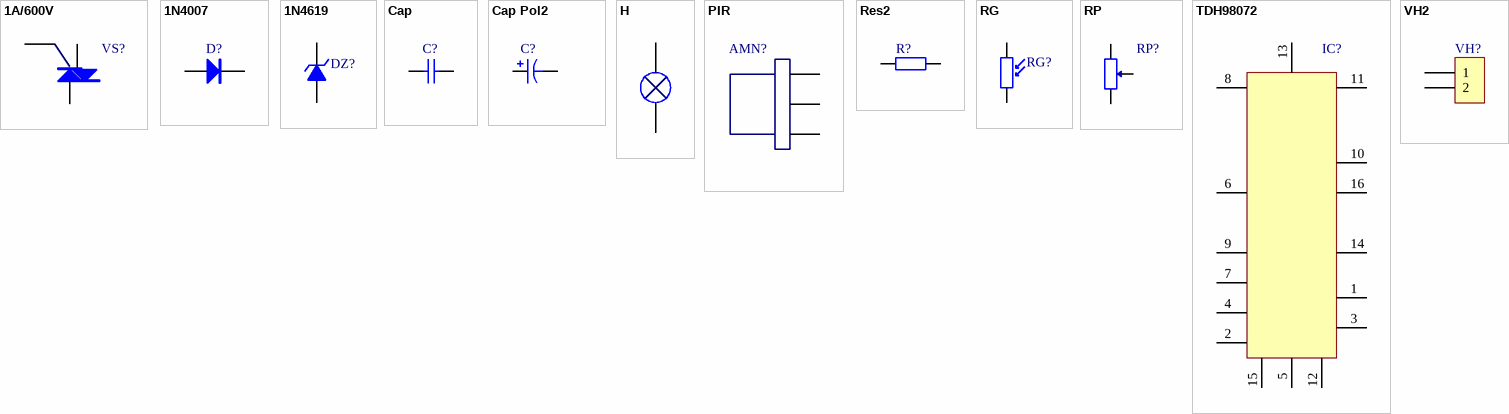
[diagram p0: symbols 1A/600V to VH2]
# Altium schematic symbol library MISC82068-5.SCHLIB: 12 symbols
Pins are listed as number, name and electrical type; pins without a type are passive.


## 1A/600V
designator VS?
footprint DO-41 (2.6*9.1mm (diameter, lead spacing))
footprint SOD-123 (2.7x1.6X1.1mm (L x W x H, excluding leads))
footprint SMA (4.5x2.6*2.2mm (L x W x H, excluding leads))
footprint DO-41V (2.6*3.5mm (diameter, lead spacing))
footprint LED 3mm-2P (3mm bicolour LED)
pins: 1, 2, 3

## 1N4007
designator D?
Rectifier diode
footprint DO-41 (2.6*9.1mm (diameter, lead spacing))
footprint SOD-123 (2.7x1.6X1.1mm (L x W x H, excluding leads))
footprint SMA (4.5x2.6*2.2mm (L x W x H, excluding leads))
footprint DO-41V (2.6*3.5mm (diameter, lead spacing))
pins: 1 A, 2 K

## 1N4619
designator DZ?
3V/0.5W Zener diode
footprint DO-35 (1.8*6.8mm (diameter, lead spacing))
footprint MINI_MELF (LL34) (1.5*3.4mm (diameter, lead spacing))
footprint DO-35V (1.8*2.5mm (diameter, lead spacing))
pins: 1 A, 2 K

## Cap
designator C?
Capacitor
footprint RAD-0.3 (Radial Cap, Thru-Hole; 2 Leads; 0.3 in Pin Spacing)
simulation model CAP (Capacitor)
signal-integrity model Cap
pins: 1, 2

## Cap Pol2
designator C?
Polarized Capacitor (Axial)
footprint POLAR0.8 (Polarized Capacitor; 2 Leads)
simulation model CAP (Capacitor)
signal-integrity model Cap Pol
pins: 1, 2
1 alternate drawing of the same symbol

## H
designator *?
footprint HDR1X2 (Connector; Header; 2 Position)
pins: 1, 2

## PIR
designator AMN?
footprint HDR1X3 (Connector; Header; 3 Position)
pins: 1, 2, 3

## Res2
designator R?
Resistor
footprint AXIAL-0.4 (Axial Device, Thru-Hole; 2 Leads; 0.4 in Pin Spacing)
simulation model RESISTOR (Resistor)
signal-integrity model Res
pins: 1, 2

## RG
designator RG?
Photoresistor
footprint RG5528 (Photoresistor, pin pitch: 3mm)
footprint AXIAL-0.4 (Axial Device, Thru-Hole; 2 Leads; 0.4 in Pin Spacing)
pins: 1, 2

## RP
designator RP?
Single potentiometer
footprint 3296W (Precise Multi-Winding Adjustable Resistor)
footprint 3306W
footprint 3319P
footprint 3362P
footprint 3386W
footprint RM065 (Blue-white adjustable potentiometer)
footprint WH148-1-G15 (Single potentiometer, pin pitch: 5mm, shaft length: 15mm)
footprint WH148-1-G18 (Single potentiometer, pin pitch: 5mm, shaft length: 18mm)
footprint WH148-1-G20 (Single potentiometer, pin pitch: 5mm, shaft length: 20mm)
footprint WH148-1-G25 (Single potentiometer, pin pitch: 5mm, shaft length: 25mm)
footprint 3266W (L: 7mm, W: 4.8mm, H: 7.5mm)
footprint 3266X (L: 7mm, W: 4.8mm, H: 7.5mm)
footprint 3266Y (L: 7mm, W: 4.8mm, H: 7.5mm)
footprint 3266Z (L: 7mm, W: 4.8mm, H: 7.5mm)
footprint XV09223NPV-20F (L 9.85mm, W 11.55mm, H 20mm)
footprint XV09223NPV-25F (L 9.85mm, W 11.55mm, H 25mm)
footprint XV09223NPV-30F (L 9.85mm, W 11.55mm, H 30mm)
footprint 3006P (19.05mm*4.83mm*6.35mm (L*W*H))
pins: 1, 2, 3

## TDH98072
designator IC?
footprint DIP16
pins: 1 VSS, 2 VSS, 3 VSS, 4 VSS, 5 VSS, 6 VSS, 7 VSS, 8 VSS, 9 VSS, 10 VSS, 11 VSS, 12 VSS, 13 VSS, 14 VSS, 15 VSS, 16 VSS

## VH2
designator VH?
footprint VH3.96-2A
footprint VH3.96-2AW
footprint VH3.96-2AWD
pins: 1, 2